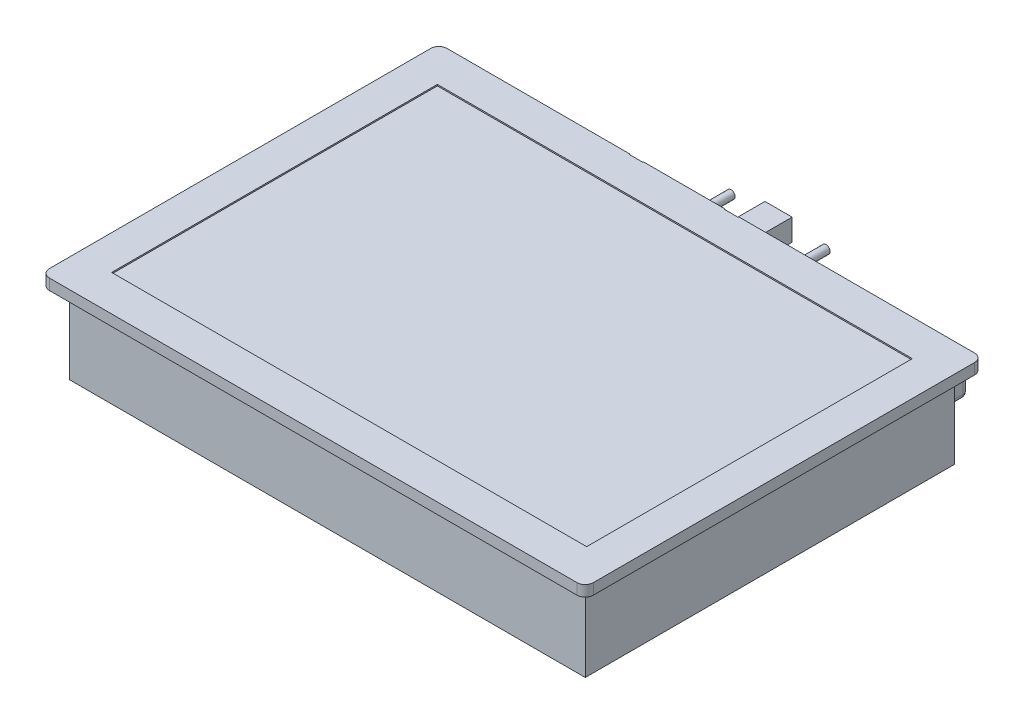
SolidWorks part; units mm, degrees
material "6061"
ref_plane "前视基准面" through (0, 0, 0) normal (0, 0, 1) x (1, 0, 0)
ref_plane "上视基准面" through (0, 0, 0) normal (0, 1, 0) x (1, 0, 0)
ref_plane "右视基准面" through (0, 0, 0) normal (1, 0, 0) x (0, 0, -1)
sketch "草图1" plane through (0, 0, 0) normal (0, 1, 0) x (1, 0, 0)
  line L1 (100.2, -73.25) -> (-100.2, -73.25)
  line L2 (100.2, -73.25) -> (100.2, 73.25)
  line L3 (100.2, 73.25) -> (-100.2, 73.25)
  line L4 (-100.2, -73.25) -> (-100.2, 73.25)
  line L5 (100.2, -73.25) -> (-100.2, 73.25) construction
  line L6 (100.2, 73.25) -> (-100.2, -73.25) construction
  point P0 (0, 0)
  dimension "D1" = 200.4
  dimension "D2" = 146.5
extrude "凸台-拉伸1" add sketch "草图1" along normal mid plane 34
sketch "草图2" plane through (0, 17, 0) normal (0, 1, 0) x (1, 0, 0)
  line L1 (-87.5, 60) -> (87.5, 60)
  line L2 (-87.5, 60) -> (-87.5, -60)
  line L3 (-87.5, -60) -> (87.5, -60)
  line L4 (87.5, 60) -> (87.5, -60)
  line L5 (-87.5, 60) -> (87.5, -60) construction
  line L6 (-87.5, -60) -> (87.5, 60) construction
  point P0 (0, 0)
  dimension "D1" = 175
  dimension "D2" = 120
extrude "切除-拉伸1" cut sketch "草图2" against normal blind 0.5
sketch "草图3" plane through (0, -17, 0) normal (0, -1, 0) x (1, 0, 0)
  line L1 (100.2, -73.25) -> (-100.2, -73.25)
  line L2 (100.2, -73.25) -> (100.2, 73.25)
  line L3 (100.2, 73.25) -> (-100.2, 73.25)
  line L4 (-100.2, -73.25) -> (-100.2, 73.25)
  line L5 (95, -68) -> (-95, -68)
  line L6 (95, -68) -> (95, 68)
  line L7 (95, 68) -> (-95, 68)
  line L8 (-95, -68) -> (-95, 68)
  line L9 (95, -68) -> (-95, 68) construction
  line L10 (95, 68) -> (-95, -68) construction
  point P6 (0, 0)
  dimension "D1" = 190
  dimension "D2" = 136
extrude "切除-拉伸2" cut sketch "草图3" against normal blind 30
fillet "圆角1" radius 3 4 edges at (100.2, 15, 73.25) (-100.2, 15, 73.25) (-100.2, 15, -73.25) (100.2, 15, -73.25)
sketch "草图4" plane through (0, 0, -68) normal (0, 0, -1) x (-1, 0, 0)
  line L1 (29.8, -16) -> (-10.2, -16)
  line L2 (29.8, -16) -> (29.8, -8)
  line L3 (29.8, -8) -> (-10.2, -8)
  line L4 (-10.2, -16) -> (-10.2, -8)
  line L5 (95, -17) -> (-95, -17) construction
  point P8 (-10.2, -12)
  dimension "D1" = 90
  dimension "D2" = 8
  dimension "D3" = 1
  dimension "D4" = 40
extrude "凸台-拉伸2" add sketch "草图4" along normal blind 40
sketch "草图5" plane through (0, 0, -68) normal (0, 0, -1) x (-1, 0, 0)
  line L0 (95, -17) -> (-95, -17) construction
  line L1 (-65.2, -13) -> (-80.2, -13)
  line L2 (-65.2, -13) -> (-65.2, -5)
  line L3 (-65.2, -5) -> (-80.2, -5)
  line L4 (-80.2, -13) -> (-80.2, -5)
  dimension "D1" = 20
  dimension "D2" = 15
  dimension "D3" = 8
  dimension "D4" = 4
extrude "凸台-拉伸3" add sketch "草图5" along normal blind 20
fillet "圆角2" radius 2 8 edges at (80.2, -9, -88) (65.2, -9, -88) (72.7, -5, -88) (72.7, -13, -88) (65.2, -5, -78) (80.2, -5, -78) (65.2, -13, -78) (80.2, -13, -78)
sketch "草图6" plane through (0, 0, -88) normal (0, 0, -1) x (-1, 0, 0)
  line L0 (-67.2, -9) -> (-78.2, -9) construction
  line L1 (-67.2, -11) -> (-67.2, -7) construction
  line L2 (-78.2, -7) -> (-78.2, -11) construction
  line L3 (-72.7, -11) -> (-72.7, -7) construction
  line L4 (-78.2, -11) -> (-67.2, -11) construction
  line L5 (-67.2, -7) -> (-78.2, -7) construction
  circle A0 centre (-72.7, -9) radius 1.75
  dimension "D1" = 3.5
extrude "凸台-拉伸4" add sketch "草图6" along normal blind 5
sketch "草图7" plane through (0, -16, 0) normal (0, -1, 0) x (1, 0, 0)
  line L0 (-29.8, -88) -> (-19.8, -88)
  line L2 (-29.8, -108) -> (-29.8, -68) construction
  line L3 (-19.8, -88) -> (-14.8, -98)
  line L4 (-14.8, -98) -> (-14.8, -108)
  line L5 (10.2, -108) -> (-29.8, -108) construction
  line L6 (-14.8, -108) -> (-29.8, -108)
  line L7 (-29.8, -108) -> (-29.8, -88)
  line L8 (-9.8, -108) -> (-9.8, -59.4643) construction
  line L9 (-4.8, -98) -> (-4.8, -108)
  line L10 (-4.8, -98) -> (0.2, -88)
  line L11 (0.2, -88) -> (10.2, -88)
  line L12 (10.2, -108) -> (10.2, -68) construction
  line L13 (10.2, -88) -> (10.2, -108)
  line L14 (10.2, -108) -> (-4.8, -108)
  point P12 (-4.8, -103)
  dimension "D1" = 5
  dimension "D2" = 10
  dimension "D3" = 20
  dimension "D4" = 10
  dimension "D5" = 20
  dimension "D6" = 10
  dimension "D7" = 5
  dimension "D8" = 10
extrude "切除-拉伸3" cut sketch "草图7" against normal through all
sketch "草图8" plane through (0, -16, 0) normal (0, -1, 0) x (1, 0, 0)
  line L1 (-29.8, -88) -> (-24.8, -88)
  line L2 (-29.8, -88) -> (-29.8, -73)
  line L3 (-29.8, -73) -> (-24.8, -73)
  line L4 (-24.8, -88) -> (-24.8, -73)
  line L5 (10.2, -88) -> (5.2, -88)
  line L6 (10.2, -88) -> (10.2, -73)
  line L7 (10.2, -73) -> (5.2, -73)
  line L8 (5.2, -88) -> (5.2, -73)
  dimension "D1" = 5
  dimension "D2" = 5
  dimension "D3" = 15
  dimension "D4" = 15
extrude "切除-拉伸4" cut sketch "草图8" against normal through all
sketch "草图9" plane through (0, 0, -73) normal (0, 0, -1) x (-1, 0, 0)
  line L0 (29.8, -12) -> (-10.2, -12) construction
  line L1 (29.8, -8) -> (29.8, -16) construction
  line L2 (-10.2, -8) -> (-10.2, -16) construction
  line L3 (9.8, -12) -> (9.8, 65.6604) construction
  circle A0 centre (27.3, -12) radius 1.5
  circle A1 centre (-7.7, -12) radius 1.5
  dimension "D1" = 35
  dimension "D2" = 3
extrude "凸台-拉伸5" add sketch "草图9" along normal blind 35
